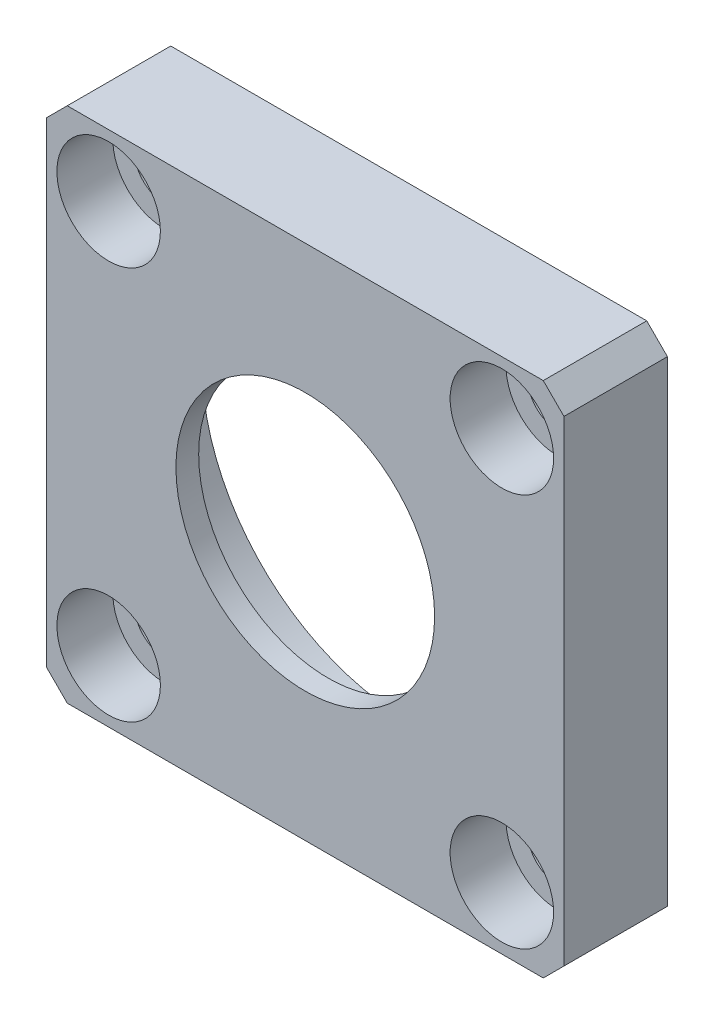
from build123d import *

# Parameters (mm, degrees)
SKETCH_1_W                   = 50
SKETCH_1_H                   = 50
EXTRUDE_1_DEPTH              = 5
SKETCH_2_R                   = 20
CUT_EXTRUDE_1_DEPTH          = 37.742346142
HOLE_WIZARD_M5_1_D           = 5.8
HOLE_WIZARD_M5_1_CBORE_D     = 10
HOLE_WIZARD_M5_1_CBORE_DEPTH = 5.4
CHAMFER_1_SIZE               = 2
SKETCH_7_R                   = 20
SKETCH_7_R_2                 = 12.5
EXTRUDE_2_DEPTH              = 2.2


with BuildPart() as part:
    # 草图1 → 凸台-拉伸1 (new, symmetric)
    with BuildSketch(Plane.XY):
        Rectangle(SKETCH_1_W, SKETCH_1_H)
    extrude(amount=EXTRUDE_1_DEPTH, both=True)

    # 草图2 → 切除-拉伸1 (cut, through all)
    with BuildSketch(Plane.XY.offset(5)):
        Circle(SKETCH_2_R)
    extrude(amount=-CUT_EXTRUDE_1_DEPTH, mode=Mode.SUBTRACT)

    # M5 六角凹头螺钉的柱形沉头孔1 (through all)
    with Locations(Plane.XY.offset(5)):
        with Locations((-19, 19), (19, 19), (-19, -19), (19, -19)):
            CounterBoreHole(HOLE_WIZARD_M5_1_D / 2, HOLE_WIZARD_M5_1_CBORE_D / 2, HOLE_WIZARD_M5_1_CBORE_DEPTH)

    # 倒角1
    chamfer_1_edges = [part.edges().sort_by_distance(p)[0] for p in [
        (25, -25, 0),
        (-25, -25, 0),
        (-25, 25, 0),
        (25, 25, 0),
    ]]
    chamfer(chamfer_1_edges, length=CHAMFER_1_SIZE)

    # 草图7 → 凸台-拉伸2 (add)
    with BuildSketch(Plane.XY.offset(5)):
        Circle(SKETCH_7_R)
        Circle(SKETCH_7_R_2, mode=Mode.SUBTRACT)
    extrude(amount=-EXTRUDE_2_DEPTH)


solid = part.part
